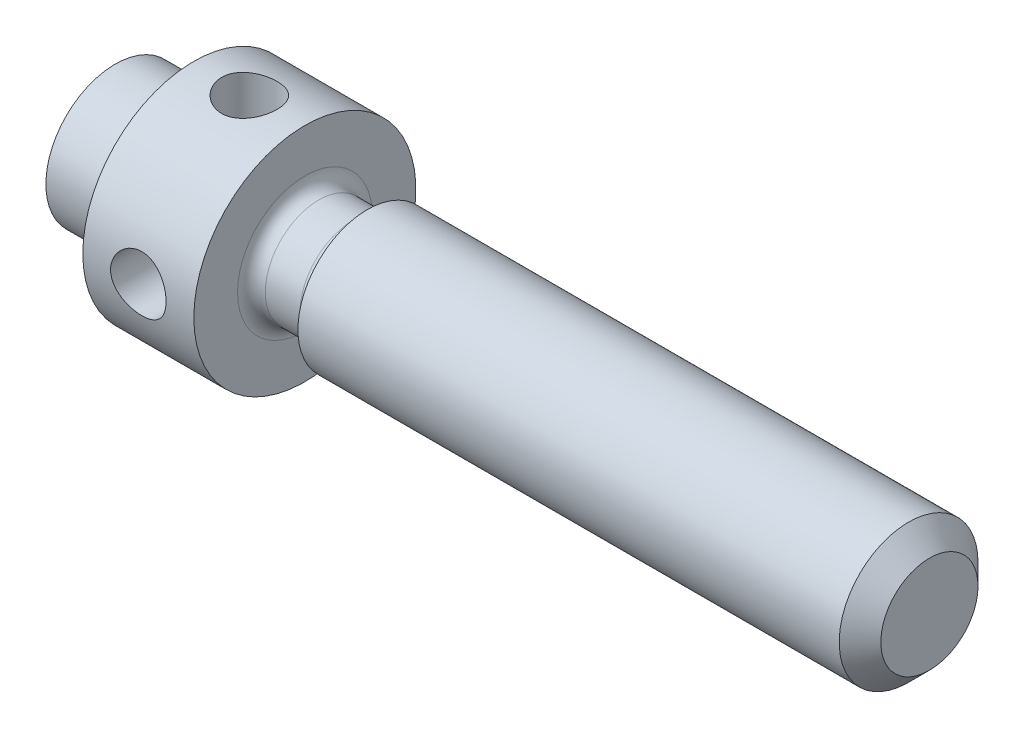
from build123d import *

# Parameters (mm, degrees)
SKETCH1_R               = 5
BOSS_EXTRUDE_DEPTH      = 40.5
CHAMFER2_SIZE           = 1.5
SKETCH2_R               = 3.85
BOSS_EXTRUDE1_DEPTH     = 4.5
SKETCH4_R               = 8
BOSS_EXTRUDE2_DEPTH     = 8
CUT_EXTRUDE1_DEPTH      = 55.194095619
CUT_EXTRUDE1_DEPTH_BACK = 55.194095619
SKETCH6_R               = 2
CUT_EXTRUDE2_DEPTH      = 55.194095747
CUT_EXTRUDE2_DEPTH_BACK = 55.194095747
SKETCH7_R               = 2
FILLET1_R               = 1
SKETCH15_W              = 10.32482264
SKETCH15_H              = 14.834361989
CUT_EXTRUDE3_DEPTH      = 21.5


with BuildPart() as part:
    # Sketch1 → Boss-Extrude (new body)
    with BuildSketch(Plane(origin=(0, 0, 0), x_dir=(0, 0, -1), z_dir=(1, 0, 0))):
        Circle(SKETCH1_R)
    extrude(amount=-BOSS_EXTRUDE_DEPTH)

    # Chamfer2
    chamfer2_edges = [part.edges().sort_by_distance(p)[0] for p in [
        (0, 0, 5),
    ]]
    chamfer(chamfer2_edges, length=CHAMFER2_SIZE)

    # Sketch2 → Boss-Extrude1 (add)
    with BuildSketch(Plane.ZY.offset(40.5)):
        with Locations(Location((0, 0, 0), (0, 0, 180))):
            Circle(SKETCH2_R)
    extrude(amount=BOSS_EXTRUDE1_DEPTH)

    # Sketch4 → Boss-Extrude2 (add)
    with BuildSketch(Plane.ZY.offset(45)):
        Circle(SKETCH4_R)
    extrude(amount=BOSS_EXTRUDE2_DEPTH)

    # Sketch6 → Cut-Extrude1 (cut, two sides: drawn at the far end of the back side and taken through both)
    with BuildSketch(Plane.XY.offset(-CUT_EXTRUDE1_DEPTH_BACK)):
        with Locations((-49, 0)):
            Circle(SKETCH6_R)
    extrude(amount=CUT_EXTRUDE1_DEPTH + CUT_EXTRUDE1_DEPTH_BACK, mode=Mode.SUBTRACT)

    # Sketch7 → Cut-Extrude2 (cut, two sides: drawn at the far end of the back side and taken through both)
    with BuildSketch(Plane(origin=(0, 0, 0), x_dir=(1, 0, 0), z_dir=(0, 1, 0)).offset(-CUT_EXTRUDE2_DEPTH_BACK)):
        with Locations(Location((-49, 0, 0), (0, 0, 270))):
            Circle(SKETCH7_R)
    extrude(amount=CUT_EXTRUDE2_DEPTH + CUT_EXTRUDE2_DEPTH_BACK, mode=Mode.SUBTRACT)

    # Sketch14 → Boss-Revolve1 (revolve)
    with BuildSketch(Plane.XY):
        with BuildLine():
            Line((-53, 0), (-53, 5))
            Line((-53, 5), (-58.660254038, 5))
            ThreePointArc((-58.660254038, 5), (-59.659258263, 2.588190451), (-60, 0))
            Line((-60, 0), (-53, 0))
        make_face()
    revolve(axis=Axis((-53, 0, 0), (-1, 0, 0)))

    # Fillet1
    fillet1_edges = [part.edges().sort_by_distance(p)[0] for p in [
        (-40.5, 0, 3.85),
        (-45, 0, 3.85),
    ]]
    fillet(fillet1_edges, radius=FILLET1_R)

    # Sketch15 → Cut-Extrude3 (cut, symmetric)
    with BuildSketch(Plane(origin=(0, 0, 0), x_dir=(1, 0, 0), z_dir=(0, 1, 0))):
        with Locations((-63.822665358, -2.417180995)):
            Rectangle(SKETCH15_W, SKETCH15_H)
    extrude(amount=CUT_EXTRUDE3_DEPTH, both=True, mode=Mode.SUBTRACT)


solid = part.part
